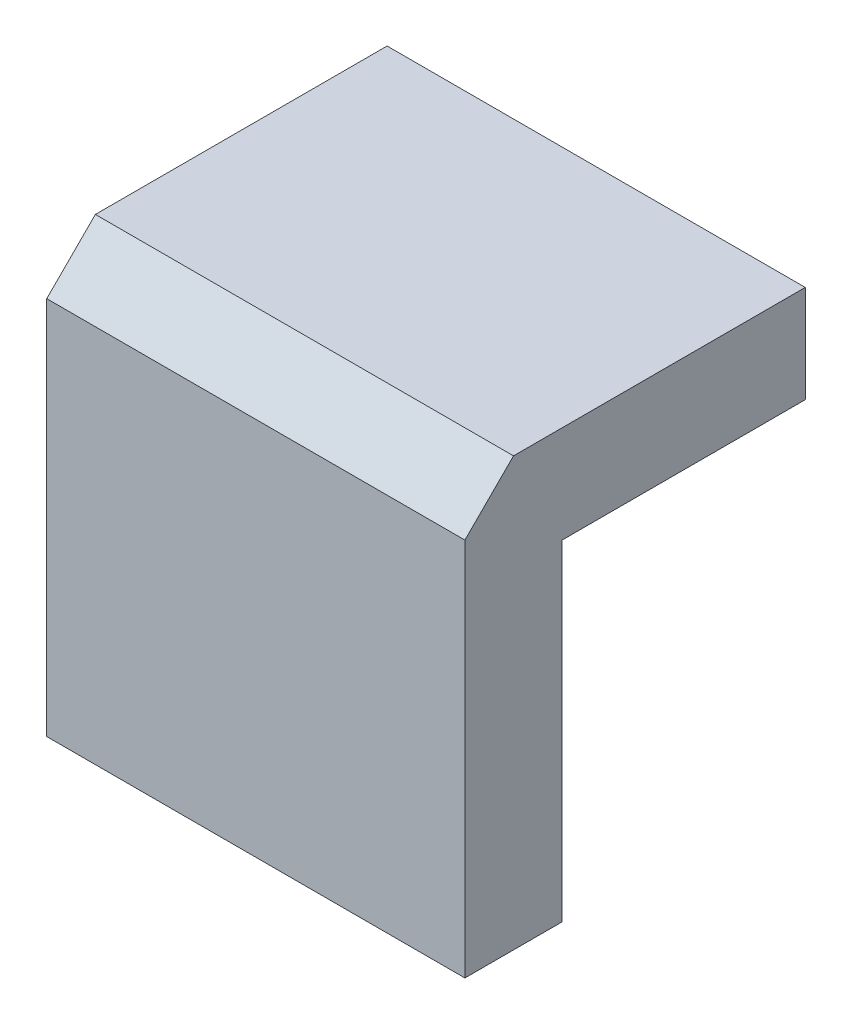
SolidWorks part; units mm, degrees
material "6061 合金"
ref_plane "前视基准面" through (0, 0, 0) normal (0, 0, 1) x (1, 0, 0)
ref_plane "上视基准面" through (0, 0, 0) normal (0, 1, 0) x (1, 0, 0)
ref_plane "右视基准面" through (0, 0, 0) normal (1, 0, 0) x (0, 0, -1)
sketch "草图1" plane through (0, 0, 0) normal (0, 0, 1) x (1, 0, 0)
  line L1 (-21.5, 22) -> (21.5, 22)
  line L2 (-21.5, 22) -> (-21.5, -22)
  line L3 (-21.5, -22) -> (21.5, -22)
  line L4 (21.5, 22) -> (21.5, -22)
  line L5 (-21.5, 22) -> (21.5, -22) construction
  line L6 (-21.5, -22) -> (21.5, 22) construction
  point P0 (0, 0)
  dimension "D1" = 43
  dimension "D2" = 44
extrude "凸台-拉伸1" add sketch "草图1" along normal mid plane 35
sketch "草图2" plane through (21.5, 0, 0) normal (1, 0, 0) x (0, 0, -1)
  line L0 (-17.5, -22) -> (-17.5, 22) construction
  line L1 (42.5, -56) -> (-7.5, -56)
  line L2 (42.5, -56) -> (42.5, 12)
  line L3 (42.5, 12) -> (-7.5, 12)
  line L4 (-7.5, -56) -> (-7.5, 12)
  line L5 (42.5, -56) -> (-7.5, 12) construction
  line L6 (42.5, 12) -> (-7.5, -56) construction
  line L7 (-17.5, 22) -> (17.5, 22) construction
  point P0 (17.5, -22)
  dimension "D1" = 10
  dimension "D2" = 10
extrude "切除-拉伸1" cut sketch "草图2" against normal through all
hole_wizard "M4 螺纹孔1" positions "草图4" profile "草图3" tap size "M4" standard "GB"
sketch "草图4" plane through (0, 0, -17.5) normal (0, 0, -1) x (-1, 0, 0)
  line L0 (-15, 17) -> (15, 17) construction
  line L3 (0, 17) -> (0, 0) construction
  line L6 (-15, 17) -> (-21.5, 17) construction
  line L7 (-21.5, 12) -> (-21.5, 22) construction
  point P0 (-15, 17)
  point P2 (15, 17)
  dimension "D1" = 30
sketch "草图3" plane through (15, 17, -17.5) normal (1, 0, 0) x (0, 1, 0)
  line L0 (0, 0) -> (0, 16.4914)
  line L1 (0, 16.4914) -> (1.65, 15.5)
  line L2 (1.65, 15.5) -> (1.65, 0)
  line L5 (1.65, 0) -> (0, 0)
  line L10 (0, 16.4914) -> (-1.65, 15.5) construction
  line L11 (0, -6.35) -> (0, 107.95) construction
  dimension "螺纹孔钻头直径" = 3.3
  dimension "螺纹孔钻头深度" = 15.5
  dimension "导头角度" = 118
cosmetic thread "孔螺蚊线1" parameters "D1"=12, "D2"=4
cosmetic thread "孔螺蚊线2" parameters "D1"=12, "D2"=4
chamfer "倒角1" distance 5 angle 45 1 edges at (0, 22, 17.5)
hole_wizard "M4 螺纹孔2" positions "草图6" profile "草图5" tap size "M4" standard "GB"
sketch "草图6" plane through (0, -22, 0) normal (0, -1, 0) x (-1, 0, 0)
  line L0 (10, -12.5) -> (-10, -12.5) construction
  line L1 (-10, -12.5) -> (-21.5, -12.5) construction
  line L4 (0, -12.5) -> (0, 0) construction
  point P0 (10, -12.5)
  point P2 (-10, -12.5)
  dimension "D1" = 20
sketch "草图5" plane through (-10, -22, 12.5) normal (1, 0, 0) x (0, 0, -1)
  line L0 (0, 0) -> (0, 16.4914)
  line L1 (0, 16.4914) -> (1.65, 15.5)
  line L2 (1.65, 15.5) -> (1.65, 0)
  line L5 (1.65, 0) -> (0, 0)
  line L10 (0, 16.4914) -> (-1.65, 15.5) construction
  line L11 (0, -6.35) -> (0, 107.95) construction
  dimension "螺纹孔钻头直径" = 3.3
  dimension "螺纹孔钻头深度" = 15.5
  dimension "导头角度" = 118
cosmetic thread "孔螺蚊线3" parameters "D1"=12, "D2"=4
cosmetic thread "孔螺蚊线4" parameters "D1"=12, "D2"=4
